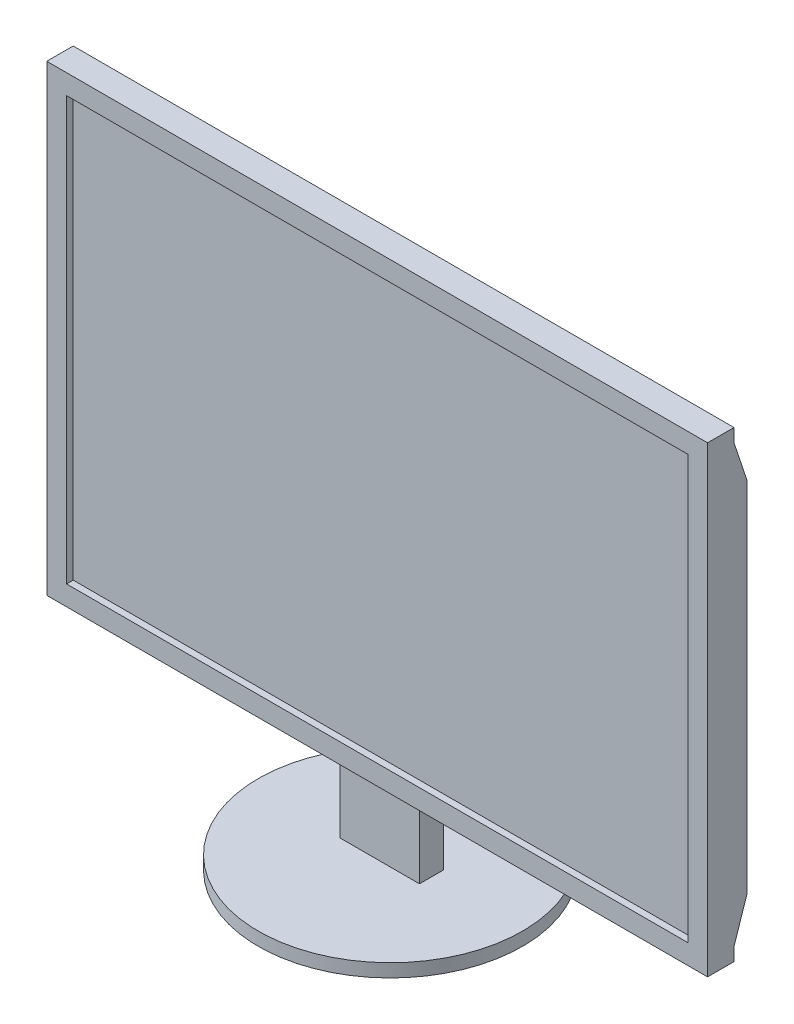
SolidWorks part; units mm, degrees
material "PBT 一般用途"
ref_plane "Front Plane" through (0, 0, 0) normal (0, 0, 1) x (1, 0, 0)
ref_plane "Top Plane" through (0, 0, 0) normal (0, 1, 0) x (1, 0, 0)
ref_plane "Right Plane" through (0, 0, 0) normal (1, 0, 0) x (0, 0, -1)
sketch "Sketch1" plane through (0, 0, 0) normal (0, 0, 1) x (1, 0, 0)
  line L1 (0, 0) -> (500, 0)
  line L2 (0, 0) -> (0, 350)
  line L3 (0, 350) -> (500, 350)
  line L4 (500, 0) -> (500, 350)
  dimension "D1" = 350
  dimension "D2" = 500
extrude "Boss-Extrude1" add sketch "Sketch1" along normal blind 20
sketch "Sketch2" plane through (500, 0, 0) normal (1, 0, 0) x (0, 0, -1)
  line L0 (0, 340) -> (0, 10)
  line L1 (0, 0) -> (0, 350) construction
  line L2 (0, 10) -> (10, 40)
  line L3 (10, 40) -> (10, 310)
  line L4 (10, 310) -> (0, 340)
  dimension "D1" = 330
  dimension "D2" = 10
  dimension "D3" = 30
  dimension "D4" = 30
  dimension "D5" = 10
extrude "Boss-Extrude2" add sketch "Sketch2" against normal blind 500
sketch "Sketch3" plane through (0, 0, 20) normal (0, 0, 1) x (1, 0, 0)
  line L0 (500, 350) -> (0, 350) construction
  line L1 (15, 335) -> (485, 335)
  line L2 (15, 335) -> (15, 15)
  line L3 (15, 15) -> (485, 15)
  line L4 (485, 335) -> (485, 15)
  line L5 (500, 0) -> (500, 350) construction
  line L6 (0, 0) -> (500, 0) construction
  line L7 (0, 350) -> (0, 0) construction
  dimension "D1" = 15
  dimension "D2" = 15
  dimension "D3" = 15
  dimension "D4" = 15
extrude "Cut-Extrude1" cut sketch "Sketch3" against normal blind 5
sketch "Sketch4" plane through (0, 0, 0) normal (0, -1, 0) x (1, 0, 0)
  line L2 (220, 18) -> (220, 0)
  line L3 (220, 0) -> (280, 0)
  line L4 (280, 18) -> (280, 0)
  line L5 (0, 0) -> (500, 0) construction
  line L6 (500, 20) -> (500, 0) construction
  line L8 (220, 18) -> (280, 18)
  dimension "D2" = 220
extrude "Boss-Extrude3" add sketch "Sketch4" along normal blind 50
sketch "Sketch5" plane through (0, -50, 0) normal (0, -1, 0) x (1, 0, 0)
  line L0 (0, 20) -> (500, 20) construction
  line L1 (280, 0) -> (280, 18) construction
  circle A0 centre (250, 10) radius 100
  dimension "D3" = 200
  dimension "D1" = 10
  dimension "D2" = 30
extrude "Boss-Extrude4" add sketch "Sketch5" along normal blind 10
